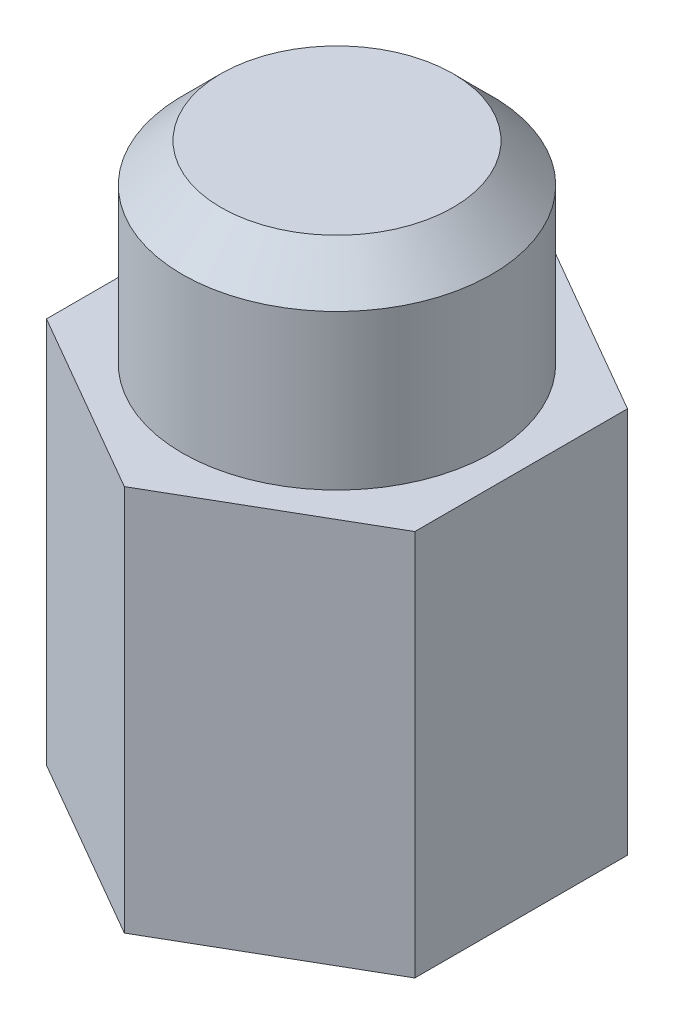
from build123d import *

# Parameters (mm, degrees)
BOSS_EXTRUDE1_DEPTH       = 5
SKETCH3_R                 = 4
BOSS_EXTRUDE2_DEPTH       = 5
CHAMFER1_SIZE             = 1
M6X1_0_TAPPED_HOLE1_D     = 5
M6X1_0_TAPPED_HOLE1_DEPTH = 8
M6X1_0_TAPPED_HOLE1_TIP   = 1.502151548


with BuildPart() as part:
    # Sketch1 → Boss-Extrude1 (new, symmetric)
    with BuildSketch(Plane(origin=(0, 0, 0), x_dir=(1, 0, 0), z_dir=(0, 1, 0))):
        Polygon((0, 5.5), (-4.763139721, 2.75), (-4.763139721, -2.75), (0, -5.5), (4.763139721, -2.75), (4.763139721, 2.75), align=None)
    extrude(amount=BOSS_EXTRUDE1_DEPTH, both=True)

    # Sketch3 → Boss-Extrude2 (add)
    with BuildSketch(Plane(origin=(0, 5, 0), x_dir=(1, 0, 0), z_dir=(0, 1, 0))):
        with Locations(Location((0, 0, 0), (0, 0, 270))):
            Circle(SKETCH3_R)
    extrude(amount=BOSS_EXTRUDE2_DEPTH)

    # Chamfer1
    chamfer1_edges = [part.edges().sort_by_distance(p)[0] for p in [
        (0, 10, -4),
    ]]
    chamfer(chamfer1_edges, length=CHAMFER1_SIZE)

    # M6x1.0 Tapped Hole1
    with Locations(Plane(origin=(0, -5, 0), x_dir=(-1, 0, 0), z_dir=(0, -1, 0))):
        with Locations((-0.001364709, 0)):
            Hole(M6X1_0_TAPPED_HOLE1_D / 2, depth=M6X1_0_TAPPED_HOLE1_DEPTH)
            with Locations((0, 0, -(M6X1_0_TAPPED_HOLE1_DEPTH + M6X1_0_TAPPED_HOLE1_TIP / 2))):  # 118° drill point
                Cone(0, M6X1_0_TAPPED_HOLE1_D / 2, M6X1_0_TAPPED_HOLE1_TIP, mode=Mode.SUBTRACT)


solid = part.part
